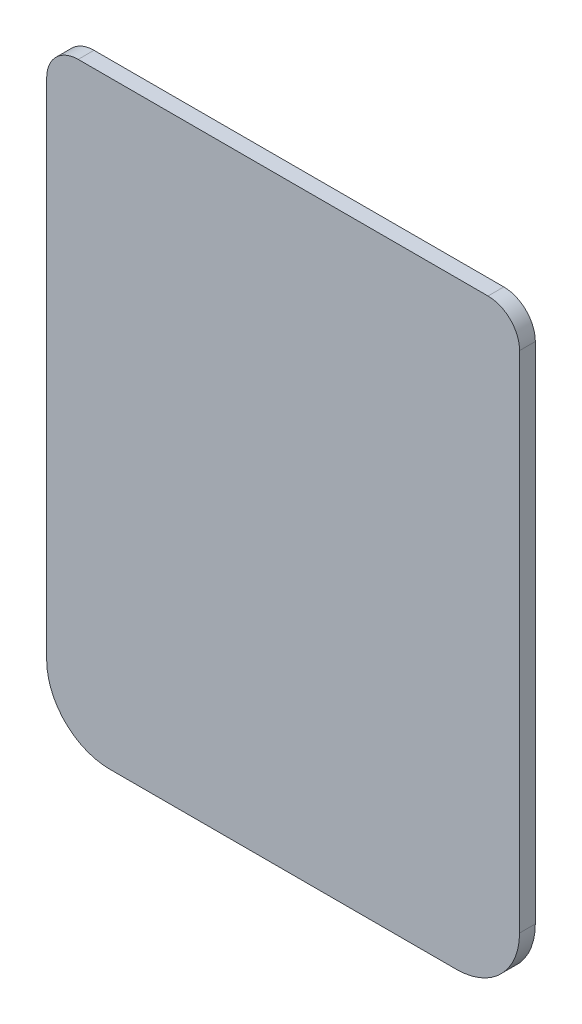
SolidWorks part; units mm, degrees
ref_plane "Front Plane" through (0, 0, 0) normal (0, 0, 1) x (1, 0, 0)
ref_plane "Top Plane" through (0, 0, 0) normal (0, 1, 0) x (1, 0, 0)
ref_plane "Right Plane" through (0, 0, 0) normal (1, 0, 0) x (0, 0, -1)
sketch "Sketch1" plane through (0, 0, 0) normal (0, 0, 1) x (1, 0, 0)
  line L1 (-75, 95) -> (75, 95)
  line L2 (-75, 95) -> (-75, -95)
  line L3 (-75, -95) -> (75, -95)
  line L4 (75, 95) -> (75, -95)
  line L5 (-75, 95) -> (75, -95) construction
  line L6 (-75, -95) -> (75, 95) construction
  point P0 (0, 0)
  dimension "D1" = 150
  dimension "D2" = 190
extrude "Boss-Extrude1" add sketch "Sketch1" along normal blind 5
fillet "Fillet1" radius 10 2 edges at (-75, 95, 2.5) (75, 95, 2.5)
fillet "Fillet2" radius 20 2 edges at (-75, -95, 2.5) (75, -95, 2.5)
